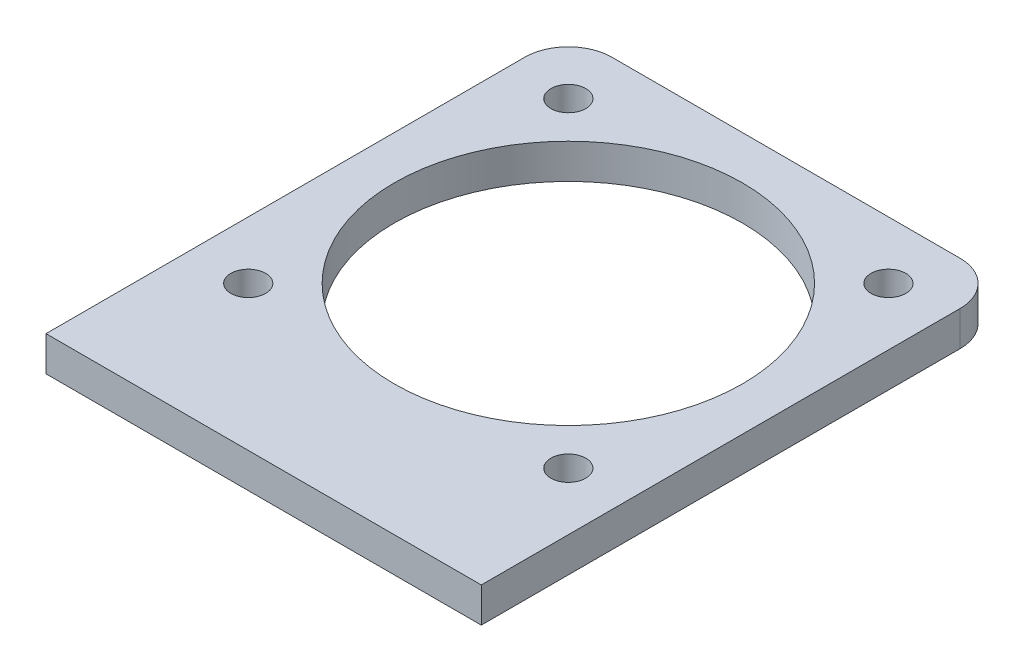
SolidWorks part; units mm, degrees
material "Q235B"
ref_plane "Front Plane" through (0, 0, 0) normal (0, 0, 1) x (1, 0, 0)
ref_plane "Top Plane" through (0, 0, 0) normal (0, 1, 0) x (1, 0, 0)
ref_plane "Right Plane" through (0, 0, 0) normal (1, 0, 0) x (0, 0, -1)
sketch "Sketch1" plane through (0, 0, 0) normal (0, 1, 0) x (1, 0, 0)
  line L1 (50, -60) -> (-50, -60)
  line L2 (50, -60) -> (50, 60)
  line L3 (50, 60) -> (-50, 60)
  line L4 (-50, -60) -> (-50, 60)
  line L5 (50, -60) -> (-50, 60) construction
  line L6 (50, 60) -> (-50, -60) construction
  point P0 (0, 0)
  dimension "D1" = 120
  dimension "D2" = 100
extrude "Boss-Extrude1" add sketch "Sketch1" along normal blind 8
fillet "Fillet1" radius 10 2 edges at (50, 4, -60) (-50, 4, -60)
sketch "Sketch2" plane through (0, 8, 0) normal (0, 1, 0) x (1, 0, 0)
  line L0 (-50, 50) -> (-50, -60) construction
  line L1 (-50, -60) -> (50, -60) construction
  circle A0 centre (0, 10) radius 40
  dimension "D1" = 80
  dimension "D2" = 50
  dimension "D3" = 70
extrude "Cut-Extrude1" cut sketch "Sketch2" against normal up to next
hole_wizard "Ø8.0 (8) Diameter Hole1" positions "Sketch3" profile "Sketch4" hole size "Ø8.0" standard "GB" end condition up to next
sketch "Sketch3" plane through (0, 8, 0) normal (0, 1, 0) x (1, 0, 0)
  line L0 (0, 10) -> (-36.7696, 46.7696) construction
  circle A0 centre (0, 10) radius 52 construction
  point P0 (-36.7696, 46.7696)
  dimension "D1" = 104
  dimension "D2" = 45
sketch "Sketch4" plane through (-36.7696, 8, -46.7696) normal (1, 0, 0) x (0, 0, 1)
  line L0 (0, 0) -> (0, 8)
  line L1 (0, 8) -> (4, 8)
  line L2 (4, 8) -> (4, 0)
  line L5 (4, 0) -> (0, 0)
  line L11 (0, -6.35) -> (0, 107.95) construction
  dimension "通孔孔直径" = 8
  dimension "通孔孔深度" = 8
pattern_circular "CirPattern1" count 4 over 360 about axis through (0, 0, -10) along (0, 1, 0) of "Ø8.0 (8) Diameter Hole1"
